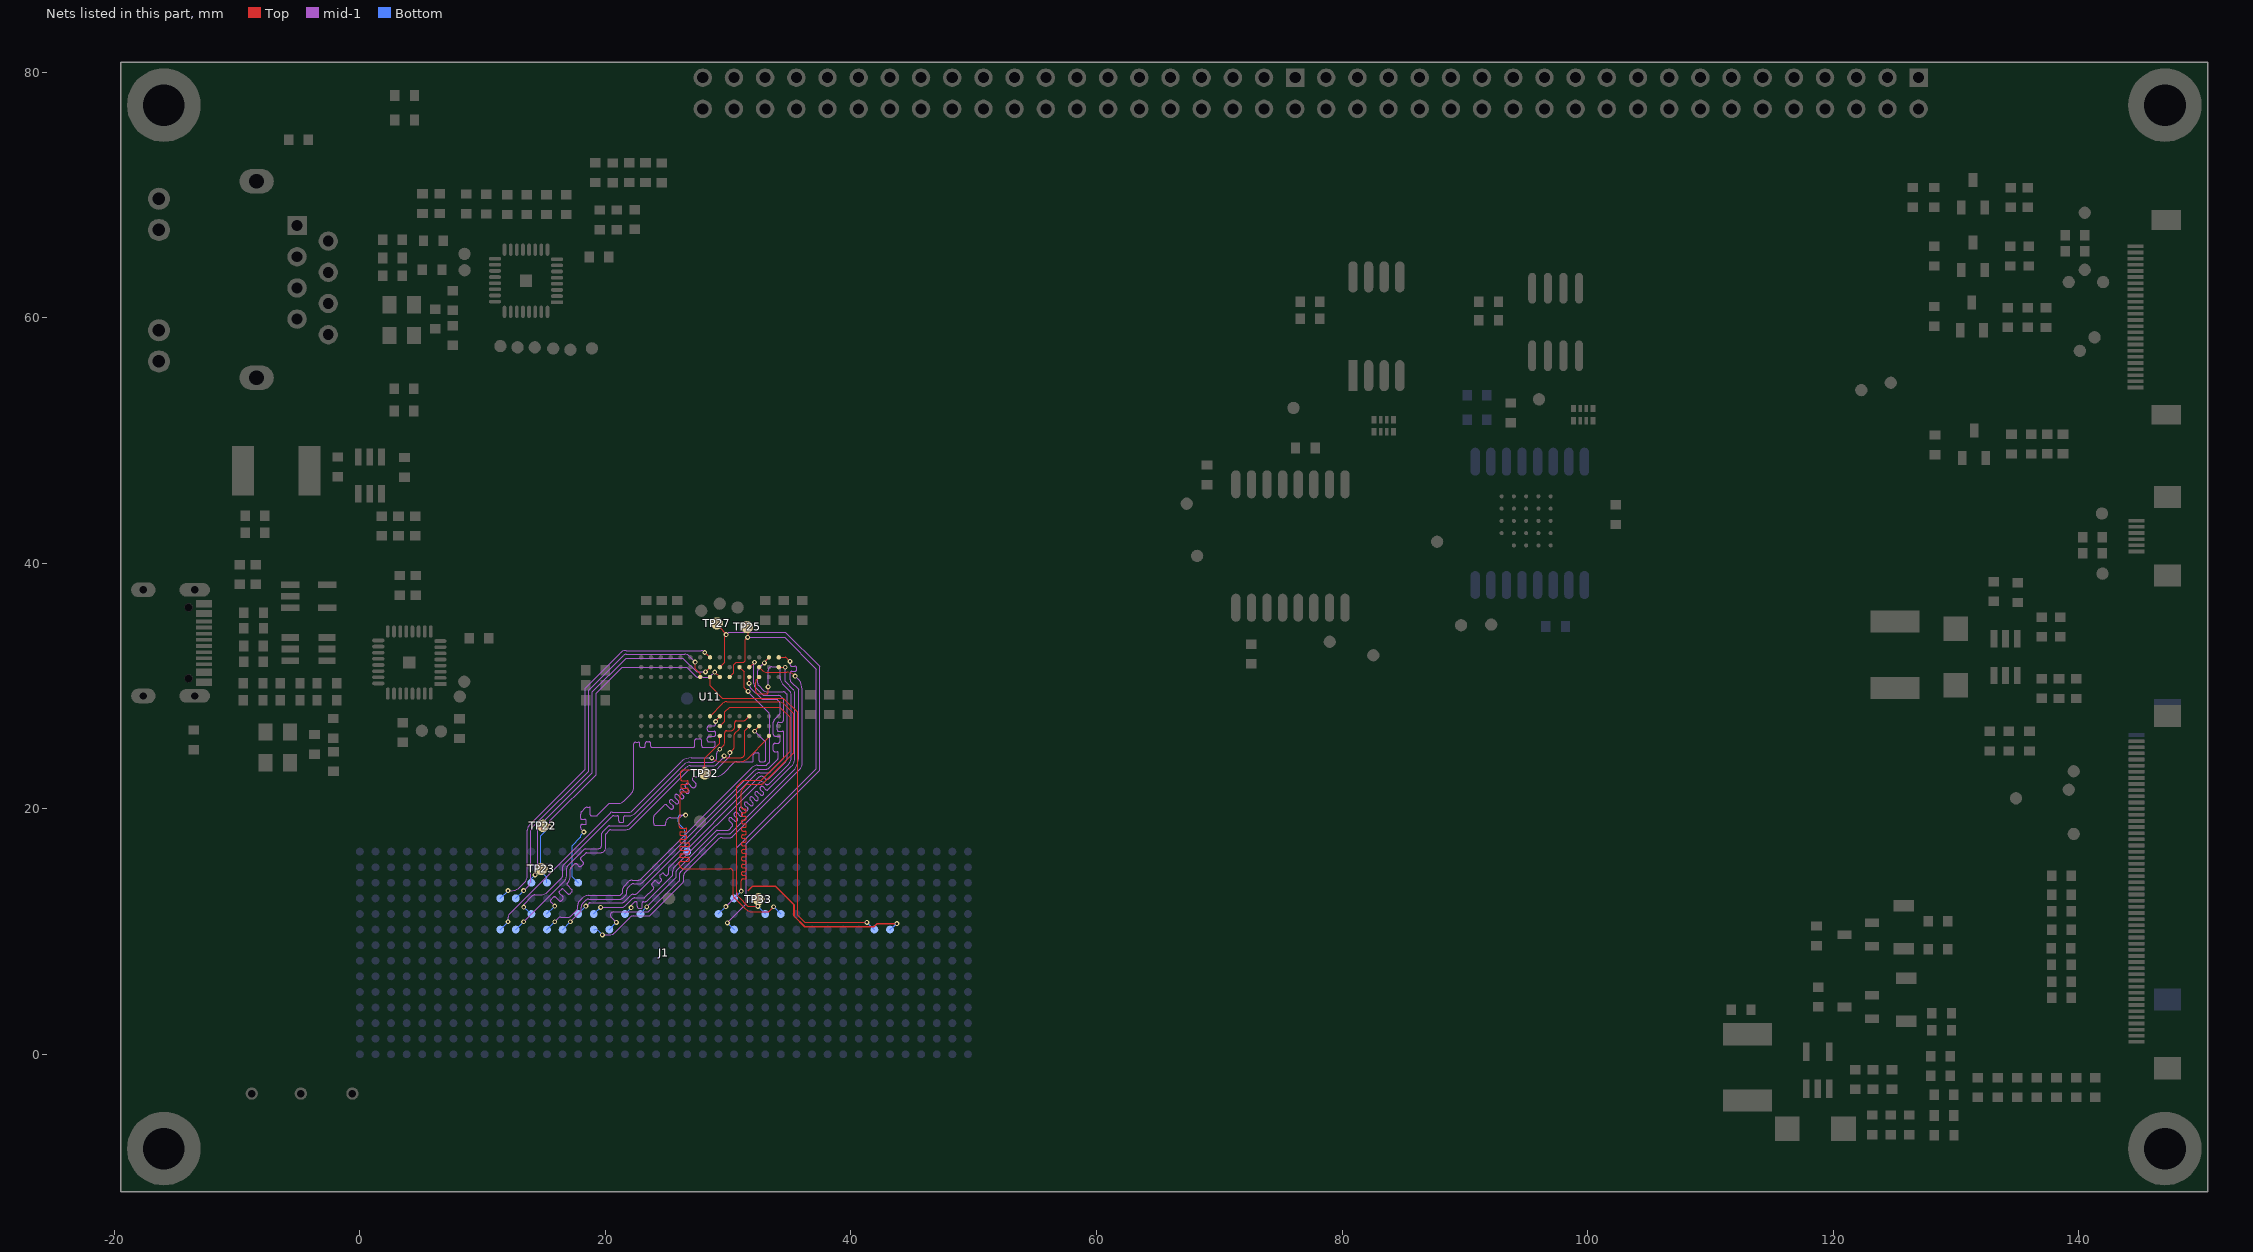
[diagram p0: the nets of this part, all layers, seen from the top]
# Altium PCB MISC105414.PcbDoc (part 9 of 11)
Units mm, origin at the board's own origin, x right, y up, seen from the top; angles counter-clockwise.
Board outline 170 x 92 mm, 6 copper layers (Top, GND, mid-1, mid-2, mid-3, Bottom), stack 1.231 mm thick; 238 components, 304 nets, 1456 pads, 1258 vias.
Unrouted connection lines stored in the file: 57.

## Via types
v1: diameter 0.4, hole 0.2, Top to Bottom, tented top, 618 vias
v2: diameter 0.5, hole 0.3, Top to Bottom, tented top, 522 vias
v3: diameter 0.5, hole 0.3, Top to Bottom, 41 vias
v4: diameter 1, hole 0.5, Top to Bottom, tented top, 36 vias
v5: diameter 0.7, hole 0.4, Top to Bottom, tented top, 34 vias
v6: diameter 1.3, hole 1.3, Top to Bottom, tented top, 3 vias
v7: diameter 4, hole 4, Top to Bottom, tented top, 2 vias
v8: diameter 3.3, hole 3.3, Top to Bottom, tented top, 2 vias

## Nets (pads, with @x,y where several pads share a name; then routed paths per layer and width w, separated by ;. In a path a pad name is that pad's centre, name@x,y a point inside that pad or via, vN(x,y) a via of type N, cw(c..) or ccw(c..) an arc to the next point about the centre after c; other vN are vias at no path point) (continued)
SDR_A9: J1.K26 U11.J3 | length 30.7
  Top w0.1: v1(28.97,27.109) U11.J3@29.32,27.533
  mid-1 w0.1: v1(18.243,18.106) 18.035,18.314 cw(c18.184,18.463) 17.973,18.463 17.973,18.604 cw(c18.094,18.604) 18.094,18.725 18.36,18.725 ccw(c18.36,18.797) 18.432,18.797 18.432,19.034 ccw(c18.334,19.034) 18.334,19.132 18.069,19.132 cw(c18.069,19.228) 17.973,19.228 17.973,19.562 cw(c18.272,19.562) 18.061,19.773 18.363,20.075 cw(c18.525,19.913) 18.525,20.142 18.678,20.142 cw(c18.678,20.044) 18.776,20.044 18.776,19.522 ccw(c18.88,19.522) 18.88,19.417 19.232,19.417 ccw(c19.232,19.57) 19.341,19.462 20.329,20.451 21.108,20.451 ccw(c21.108,21.002) 21.498,20.612 22.075,21.189 ccw(c21.507,21.758) 22.31,21.758 22.31,25.277 cw(c22.469,25.277) 22.469,25.435 22.688,25.435 cw(c22.688,25.326) 22.797,25.326 22.797,25.093 ccw(c22.896,25.093) 22.896,24.994 23.137,24.994 ccw(c23.137,25.094) 23.236,25.094 23.236,25.296 cw(c23.397,25.296) 23.397,25.456 23.546,25.456 cw(c23.546,25.317) 23.686,25.317 23.686,25.109 ccw(c23.8,25.109) 23.8,24.994 27.137,24.994 ccw(c27.137,25.14) 27.283,25.14 27.283,25.567 cw(c27.401,25.567) 27.401,25.685 27.688,25.685 cw(c27.688,25.538) 27.835,25.538 27.835,25.151 ccw(c27.992,25.151) 27.992,24.994 28.751,24.994 ccw(c28.751,25.193) 28.95,25.193 28.95,25.355 ccw(c28.853,25.355) 28.853,25.452 28.419,25.452 cw(c28.419,25.563) 28.308,25.563 28.308,25.762 cw(c28.444,25.762) 28.444,25.898 28.857,25.898 ccw(c28.857,26.011) 28.97,26.011 28.97,26.201 ccw(c28.86,26.201) 28.86,26.312 28.444,26.312 cw(c28.444,26.479) 28.277,26.479 28.277,26.609 cw(c28.425,26.609) 28.425,26.757 28.844,26.757 ccw(c28.844,26.884) 28.97,26.884 v1(28.97,27.109)
  Bottom w0.1: J1.K26@17.78,13.97 17.284,14.466 17.284,17.007 17.957,17.68 ccw(c17.842,17.794) 18.005,17.794 18.005,17.82 cw(c18.12,17.82) 18.038,17.901 v1(18.243,18.106)
SDR_A10: J1.J30 U11.G7 | length 30.9
  Top w0.1: v1(27.307,31.952) 27.307,31.398 27.72,30.985 U11.G7@27.72,30.733
  mid-1 w0.1: v1(13.335,13.335) 13.695,13.695 ccw(c13.13,14.26) 13.929,14.26 13.929,18.236 cw(c14.216,18.236) 14.014,18.439 18.647,23.072 18.647,29.663 21.475,32.491 cw(c21.705,32.261) 21.705,32.587 26.465,32.587 cw(c26.465,32.087) 26.818,32.44 v1(27.307,31.952)
  Bottom w0.1: J1.J30@12.7,12.7 v1(13.335,13.335)
SDR_A11: J1.J31 U11.H9 | length 31.9
  Top w0.1: v1(28.094,32.727) U11.H9@28.52,32.333
  mid-1 w0.1: v1(12.065,13.335) 12.404,13.335 ccw(c12.404,14.175) 12.998,13.581 13.43,14.013 ccw(c12.955,14.488) 13.627,14.488 13.627,18.233 cw(c14.219,18.233) 13.8,18.652 18.346,23.198 18.346,29.816 21.208,32.678 cw(c21.717,32.169) 21.717,32.888 27.792,32.888 cw(c27.792,32.547) 28.033,32.788 v1(28.094,32.727)
  Bottom w0.1: J1.J31@11.43,12.7 v1(12.065,13.335)
SDR_A12: J1.G6 J1.J16 U11.H3 | length 46.1
  Top w0.1: U11.H3@28.52,27.533 29.574,28.586 cw(c29.895,28.265) 29.895,28.72 34.071,28.72 cw(c34.071,28.042) 34.551,28.521 35.268,27.804 cw(c35.064,27.6) 35.353,27.6 35.353,24.658 cw(c35.088,24.658) 35.275,24.471 32.875,22.071 cw(c32.72,22.226) 32.72,22.006 31.644,22.006 ccw(c31.644,21.774) 31.48,21.938 31.182,21.641 ccw(c31.44,21.383) 31.075,21.383 31.075,20.131 ccw(c31.225,20.131) 31.225,19.981 31.338,19.981 cw(c31.338,19.831) 31.488,19.831 cw(c31.338,19.831) 31.338,19.681 31.225,19.681 ccw(c31.225,19.532) 31.075,19.532 ccw(c31.225,19.532) 31.225,19.382 31.338,19.382 cw(c31.338,19.231) 31.488,19.231 cw(c31.338,19.231) 31.338,19.081 31.225,19.081 ccw(c31.225,18.931) 31.075,18.931 ccw(c31.225,18.931) 31.225,18.781 31.338,18.781 cw(c31.338,18.631) 31.488,18.631 cw(c31.338,18.631) 31.338,18.481 31.225,18.481 ccw(c31.225,18.332) 31.075,18.332 ccw(c31.225,18.332) 31.225,18.182 31.338,18.182 cw(c31.338,18.032) 31.488,18.032 cw(c31.338,18.032) 31.338,17.882 31.225,17.881 ccw(c31.225,17.731) 31.075,17.731 ccw(c31.225,17.731) 31.225,17.581 31.338,17.581 cw(c31.338,17.431) 31.488,17.431 cw(c31.338,17.431) 31.338,17.281 31.225,17.281 ccw(c31.225,17.131) 31.075,17.131 ccw(c31.225,17.131) 31.225,16.982 31.338,16.982 cw(c31.338,16.832) 31.488,16.832 cw(c31.338,16.832) 31.338,16.682 31.225,16.681 ccw(c31.225,16.531) 31.075,16.531 ccw(c31.225,16.531) 31.225,16.381 31.338,16.381 cw(c31.338,16.231) 31.488,16.231 cw(c31.338,16.231) 31.338,16.081 31.225,16.081 ccw(c31.225,15.931) 31.075,15.931 ccw(c31.225,15.931) 31.225,15.782 31.338,15.782 cw(c31.338,15.632) 31.488,15.632 cw(c31.338,15.632) 31.338,15.482 31.225,15.482 ccw(c31.225,15.331) 31.075,15.331 ccw(c31.225,15.331) 31.225,15.181 31.338,15.181 cw(c31.338,15.031) 31.488,15.031 cw(c31.338,15.031) 31.338,14.881 31.225,14.881 ccw(c31.225,14.731) 31.075,14.731 ccw(c31.225,14.731) 31.225,14.581 31.338,14.581 cw(c31.338,14.432) 31.488,14.432 cw(c31.338,14.432) 31.338,14.282 31.217,14.282 ccw(c31.217,14.131) 31.067,14.131 v1(31.067,13.287)
  Top w0.127: 31.624,13.316 32.006,13.699 33.843,13.699 35.362,12.18 35.362,11.268 36.247,10.383 41.869,10.383 42.124,10.638 v1(43.746,10.638)
  Bottom w0.1: J1.J16@30.48,12.7 v1(31.067,13.287)
  Bottom w0.127: J1.G6@43.18,10.16 v1(43.746,10.638)
SDR_A13: J1.G7 U11.H7 | length 32
  Top w0.1: U11.H7@28.52,30.733 28.52,30.008 29.508,29.02 34.477,29.02 35.653,27.845 35.653,11.317 36.223,10.747 v1(41.3,10.747)
  Bottom w0.1: v1(41.3,10.747) J1.G7@41.91,10.16
SDR_BA0: J1.K28 TP22.1 U11.J7 | length 29.1
  Top w0.1: v1(28.905,31.129) U11.J7@29.32,30.733
  mid-1 w0.1: v1(15.483,18.53) 15.483,19.026 19.247,22.79 19.247,29.395 21.363,31.511 26.611,31.511 27.297,30.825 ccw(c27.547,31.075) 27.547,30.721 28.305,30.721 ccw(c28.305,31.184) 28.633,30.857 v1(28.905,31.129)
  Bottom w0.1: J1.K28@15.24,13.97 15.24,14.418 14.741,14.917 14.741,17.787 v1(15.483,18.53)
SDR_BA1: J1.K29 TP23.1 U11.H8 | length 29
  Top w0.1: v1(28.153,31.148) U11.H8@28.52,31.533
  mid-1 w0.1: v1(14.28,14.614) 14.363,14.698 14.493,14.828 14.493,18.485 18.947,22.939 18.947,29.537 21.689,32.28 26.315,32.28 27.447,31.148 v1(28.153,31.148)
  Bottom w0.1: J1.K29@13.97,13.97 13.97,14.305 v1(14.28,14.614)
SDR_CAS: J1.H17 TP25.1 U11.K7 | length 34.9
  Top w0.1: U11.K7@30.12,30.733 30.468,31.081 30.468,31.736 30.665,31.933 31.263,31.933 31.377,32.046 31.377,33.753 v1(31.576,33.952) TP25.1@31.545,34.807
  mid-1 w0.1: v1(29.807,12.022) 30.714,12.928 30.714,16.815 37.171,23.273 37.171,31.369 34.588,33.952 v1(31.576,33.952)
  Bottom w0.1: J1.H17@29.21,11.43 v1(29.807,12.022)
SDR_CKE: J1.H14 TP33.1 U11.J2 | length 27.2
  Top w0.1: U11.J2@29.32,26.733 29.314,26.734 29.72,27.14 29.72,27.896 30.112,28.288 34.2,28.288 35.05,27.437 35.05,24.67 32.78,22.4 cw(c32.554,22.626) 32.554,22.306 31.215,22.306 30.717,21.809 30.717,13.182 ccw(c31.28,13.182) 30.882,12.783 31.568,12.097 ccw(c31.697,12.227) 31.697,12.044 v1(32.421,12.044)
  Bottom w0.1: v1(32.421,12.044) 32.416,12.039 J1.H14@33.02,11.43
SDR_CLK: J1.H13 TP32.1 U11.J1 | length 32.3
  Top w0.1: U11.J1@29.32,25.933 29.32,25.347 28.093,24.121 28.093,23.483 27.789,23.179 26.283,23.179 26.127,23.023 26.127,22.43 ccw(c26.277,22.43) 26.277,22.28 26.65,22.28 cw(c26.65,22.171) 26.758,22.171 26.758,22.114 cw(c26.624,22.114) 26.624,21.98 26.277,21.98 ccw(c26.277,21.83) 26.127,21.83 ccw(c26.277,21.83) 26.277,21.68 26.644,21.68 cw(c26.644,21.557) 26.767,21.557 26.767,21.493 cw(c26.653,21.493) 26.653,21.38 26.277,21.38 ccw(c26.277,21.23) 26.127,21.23 26.114,21.216 26.114,19.373 26.004,19.264 26.004,18.582 ccw(c26.154,18.582) 26.154,18.432 26.534,18.432 cw(c26.534,18.328) 26.639,18.328 26.639,18.246 cw(c26.525,18.246) 26.525,18.132 26.194,18.132 ccw(c26.194,17.982) 26.044,17.982 ccw(c26.194,17.982) 26.194,17.832 26.527,17.832 cw(c26.527,17.739) 26.62,17.739 26.62,17.643 cw(c26.51,17.643) 26.51,17.532 26.194,17.532 ccw(c26.194,17.382) 26.044,17.382 ccw(c26.194,17.382) 26.194,17.232 26.704,17.232 cw(c26.704,17.082) 26.854,17.082 cw(c26.704,17.082) 26.704,16.932 26.194,16.932 ccw(c26.194,16.782) 26.044,16.782 ccw(c26.194,16.782) 26.194,16.632 26.704,16.632 cw(c26.704,16.482) 26.854,16.482 cw(c26.704,16.482) 26.704,16.332 26.194,16.332 ccw(c26.194,16.182) 26.044,16.182 ccw(c26.194,16.182) 26.194,16.032 26.704,16.032 cw(c26.704,15.882) 26.854,15.882 cw(c26.704,15.882) 26.704,15.732 26.182,15.732 ccw(c26.182,15.582) 26.032,15.582 26.032,15.435 ccw(c26.337,15.435) 26.337,15.13 30.11,15.13 cw(c30.11,14.823) 30.416,14.823 30.416,12.953 ccw(c30.728,12.953) 30.507,12.732 31.404,11.835 ccw(c31.933,12.364) 31.933,11.616 33.207,11.616 ccw(c33.207,11.841) 33.366,11.682 v1(33.7,12.017)
  Bottom w0.1: v1(33.7,12.017) J1.H13@34.29,11.43
SDR_CS: J1.G16 TP27.1 U11.J8 | length 37.7
  Top w0.1: TP27.1@29.077,35.099 v1(29.828,34.179) 29.713,34.064 29.713,31.926 U11.J8@29.32,31.533
  mid-1 w0.1: v1(29.828,34.179) 30.046,34.397 34.663,34.397 37.471,31.589 37.471,23.148 31.469,17.146 31.469,12.248 v1(29.932,10.711)
  Bottom w0.1: v1(29.932,10.711) J1.G16@30.48,10.16
SDR_D0: J1.H22 U11.R8 | length 33.3
  Top w0.1: U11.R8@34.12,31.533 34.128,31.525 v1(34.649,31.525)
  mid-1 w0.1: v1(23.365,12.004) 25.7,14.339 ccw(c25.54,14.5) 25.767,14.5 25.767,14.892 cw(c25.901,14.892) 25.806,14.987 29.049,18.23 cw(c29.113,18.166) 29.113,18.257 29.961,18.257 ccw(c29.961,18.41) 30.069,18.301 30.33,18.563 ccw(c30.224,18.669) 30.374,18.669 ccw(c30.224,18.669) 30.33,18.775 30.086,19.019 cw(c30.192,19.125) 30.042,19.125 cw(c30.192,19.125) 30.086,19.231 cw(c30.192,19.125) 30.298,19.231 30.516,19.014 ccw(c30.622,19.12) 30.772,19.12 ccw(c30.622,19.12) 30.728,19.226 30.511,19.443 cw(c30.617,19.55) 30.467,19.55 cw(c30.617,19.55) 30.723,19.656 30.94,19.438 ccw(c31.046,19.544) 31.196,19.544 ccw(c31.046,19.544) 31.152,19.65 30.935,19.868 cw(c31.041,19.974) 30.891,19.974 cw(c31.041,19.974) 31.147,20.08 31.364,19.862 ccw(c31.47,19.969) 31.62,19.969 ccw(c31.47,19.969) 31.576,20.075 31.359,20.292 cw(c31.465,20.398) 31.315,20.398 cw(c31.465,20.398) 31.571,20.504 31.789,20.287 ccw(c31.895,20.393) 32.045,20.393 ccw(c31.895,20.393) 32.001,20.499 31.783,20.716 cw(c31.889,20.822) 31.739,20.822 cw(c31.889,20.822) 31.995,20.928 32.213,20.711 ccw(c32.319,20.817) 32.469,20.817 ccw(c32.319,20.817) 32.425,20.923 32.208,21.141 cw(c32.314,21.247) 32.164,21.247 cw(c32.314,21.247) 32.42,21.353 32.637,21.135 ccw(c32.743,21.241) 32.893,21.241 ccw(c32.743,21.241) 32.849,21.347 32.632,21.565 cw(c32.738,21.671) 32.588,21.671 cw(c32.738,21.671) 32.844,21.777 33.061,21.56 ccw(c33.167,21.666) 33.23,21.529 35.143,23.442 ccw(c34.456,24.129) 35.428,24.129 35.428,29.381 ccw(c34.913,29.381) 35.277,29.745 34.649,30.373 v1(34.649,31.525)
  Bottom w0.1: J1.H22@22.86,11.43 22.86,11.499 v1(23.365,12.004)
SDR_D1: J1.H23 U11.N7 | length 33.4
  Top w0.1: U11.N7@32.52,30.733 32.315,30.528 ccw(c32.518,30.325) 32.231,30.325 32.231,29.607 ccw(c32.474,29.607) 32.474,29.364 33.135,29.364 ccw(c33.135,29.48) 33.251,29.48 v1(33.251,29.93)
  mid-1 w0.1: v1(22.1,11.95) 22.1,12.094 cw(c22.23,12.094) 22.138,12.185 22.329,12.376 cw(c22.488,12.216) 22.488,12.442 22.496,12.442 cw(c22.496,12.349) 22.588,12.349 22.588,12.044 ccw(c22.74,12.044) 22.74,11.892 22.899,11.892 ccw(c22.899,12.007) 23.014,12.007 23.014,12.349 cw(c23.108,12.349) 23.108,12.442 23.253,12.442 ccw(c23.253,12.589) 23.356,12.485 25.465,14.594 25.465,14.921 cw(c25.846,14.921) 25.576,15.19 ; 25.577,15.19 32.472,22.086 cw(c32.716,21.842) 32.96,22.086 33.03,22.015 ccw(c33.161,22.146) 33.292,22.015 34.914,23.637 ccw(c34.397,24.154) 35.128,24.154 35.128,29.333 ccw(c34.799,29.333) 35.031,29.566 34.412,30.186 cw(c34.809,30.583) 34.247,30.583 34.247,31.355 ccw(c34.034,31.355) 34.034,31.568 33.547,31.568 ccw(c33.547,31.273) 33.251,31.273 v1(33.251,29.93)
  Bottom w0.1: J1.H23@21.59,11.43 v1(22.1,11.95)
SDR_D2: J1.G24 U11.R9 | length 33
  Top w0.1: U11.R9@34.12,32.333 34.635,32.333 cw(c34.635,32.141) 34.77,32.277 v1(35.035,32.012)
  mid-1 w0.1: v1(20.9,10.75) 20.47,11.18 cw(c20.64,11.35) 20.399,11.35 cw(c20.64,11.35) 20.64,11.591 23.491,11.591 26.02,14.12 ccw(c25.896,14.243) 26.071,14.243 26.071,14.747 cw(c26.263,14.747) 26.127,14.883 29.162,17.918 cw(c29.256,17.823) 29.256,17.957 30.082,17.957 ccw(c30.082,18.118) 30.196,18.004 35.338,23.146 ccw(c34.397,24.087) 35.728,24.087 35.728,29.719 35.116,30.331 cw(c35.312,30.526) 35.035,30.526 35.035,31.043 cw(c35.188,31.043) 35.188,31.196 35.436,31.196 ccw(c35.436,31.342) 35.582,31.342 35.582,31.456 ccw(c35.413,31.456) 35.413,31.624 35.142,31.624 cw(c35.142,31.731) 35.035,31.731 v1(35.035,32.012)
  Bottom w0.1: J1.G24@20.32,10.16 v1(20.9,10.75)
SDR_D3: J1.G25 U11.N8 | length 33.8
  Top w0.1: U11.N8@32.52,31.533 32.764,31.289 ccw(c33.15,31.675) 33.15,31.129 34.771,31.129 cw(c34.771,30.25) 35.393,30.872 v1(35.457,30.808)
  mid-1 w0.1: v1(19.747,9.732) 20.366,9.732 ccw(c20.366,10.295) 20.763,9.897 22.035,11.168 cw(c22.269,10.934) 22.269,11.265 23.463,11.265 ccw(c23.463,11.575) 23.682,11.356 26.297,13.971 ccw(c26.112,14.156) 26.373,14.156 26.373,14.575 cw(c26.685,14.575) 26.465,14.796 29.185,17.516 cw(c29.517,17.183) 29.517,17.654 30.183,17.654 ccw(c30.183,17.873) 30.338,17.718 35.832,23.212 ccw(c35.358,23.685) 36.028,23.685 36.028,29.728 ccw(c34.8,29.728) 35.668,30.597 v1(35.457,30.808)
  Bottom w0.1: J1.G25@19.05,10.16 19.126,10.16 cw(c19.126,9.694) 19.456,10.024 v1(19.747,9.732)
SDR_D4: J1.H25 U11.P9 | length 33.2
  Top w0.1: v1(32.949,31.885) U11.P9@33.32,32.333
  mid-1 w0.1: v1(19.615,11.964) 21.301,11.964 ccw(c21.301,12.427) 21.628,12.1 22.187,12.659 cw(c22.388,12.458) 22.388,12.742 23.14,12.742 ccw(c23.14,12.86) 23.224,12.777 23.927,13.48 ccw(c23.858,13.549) 23.956,13.549 ccw(c23.858,13.549) 23.927,13.618 23.782,13.763 cw(c23.852,13.833) 23.753,13.833 cw(c23.852,13.833) 23.782,13.903 ; 23.782,13.903 23.985,14.106 cw(c24.058,14.034) 24.13,14.106 24.269,13.967 ; 24.27,13.966 ccw(c24.342,14.039) 24.413,13.966 ; 24.414,13.967 24.565,14.118 ccw(c24.49,14.194) 24.597,14.194 ccw(c24.49,14.194) 24.565,14.27 24.446,14.389 cw(c24.535,14.478) 24.409,14.478 cw(c24.535,14.478) 24.446,14.567 24.599,14.72 cw(c24.679,14.641) 24.758,14.72 24.885,14.593 ccw(c24.963,14.67) 25.04,14.593 25.125,14.678 ccw(c25.039,14.764) 25.161,14.764 25.161,15.212 32.496,22.548 cw(c32.71,22.334) 32.923,22.548 33.025,22.446 ccw(c33.162,22.582) 33.298,22.446 34.697,23.844 ccw(c34.38,24.161) 34.828,24.161 34.828,29.233 ccw(c34.69,29.233) 34.787,29.33 34.664,29.454 ; v1(32.949,31.885) 32.456,31.392 ccw(c32.602,31.246) 32.396,31.246 32.396,30.237 ccw(c32.67,30.237) 32.476,30.043 32.854,29.664 ccw(c33.18,29.99) 33.18,29.53 34.481,29.53 cw(c34.481,29.271) 34.664,29.454
  Bottom w0.1: J1.H25@19.05,11.43 19.6,11.98 v1(19.615,11.964)
SDR_D5: J1.H26 U11.M8 | length 32.9
  Top w0.1: U11.M8@31.72,31.533 v1(32.144,31.932)
  mid-1 w0.1: v1(18.415,12.065) 18.63,12.28 cw(c18.757,12.153) 18.757,12.333 21.311,12.333 ccw(c21.311,12.637) 21.526,12.422 22.061,12.957 cw(c22.283,12.735) 22.283,13.049 22.453,13.049 ccw(c22.453,13.172) 22.54,13.085 32.255,22.8 cw(c32.584,22.471) 32.584,22.937 33.26,22.937 ccw(c33.26,23.189) 33.438,23.01 34.464,24.036 ccw(c34.31,24.19) 34.528,24.19 34.528,26.2 ccw(c34.412,26.2) 34.412,26.316 34.117,26.316 cw(c34.117,26.449) 33.983,26.449 33.983,26.902 cw(c34.12,26.902) 34.12,27.039 34.31,27.039 ccw(c34.31,27.256) 34.528,27.256 34.528,28.83 ccw(c34.333,28.83) 34.471,28.967 34.309,29.129 ccw(c34.068,28.887) 34.068,29.229 32.977,29.229 cw(c32.977,29.499) 32.787,29.308 32.238,29.857 ; v1(32.144,31.932) 32.082,31.87 32.082,30.232 ccw(c32.613,30.232) 32.238,29.857
  Bottom w0.1: J1.H26@17.78,11.43 v1(18.415,12.065)
SDR_D6: J1.G27 U11.M7 | length 33.5
  Top w0.1: v1(31.702,30.217) 31.72,30.234 U11.M7@31.72,30.733
  mid-1 w0.1: v1(17.145,10.795) 17.942,11.592 ccw(c17.731,11.803) 18.029,11.803 18.029,11.99 cw(c18.474,11.99) 18.159,12.304 18.385,12.53 cw(c18.637,12.279) 18.637,12.635 21.181,12.635 ccw(c21.181,12.957) 21.409,12.729 21.694,13.014 ccw(c21.616,13.092) 21.726,13.092 21.726,13.347 cw(c22.027,13.347) 21.814,13.56 22.04,13.786 cw(c22.302,13.523) 22.302,13.894 22.796,13.894 ccw(c22.796,14.202) 23.013,13.984 32.136,23.107 cw(c32.45,22.792) 32.45,23.237 33.15,23.237 ccw(c33.15,23.455) 33.304,23.301 34.035,24.031 ccw(c33.883,24.183) 34.098,24.183 34.098,24.535 ccw(c33.979,24.535) 33.979,24.654 33.775,24.654 cw(c33.775,24.746) 33.683,24.746 33.683,25.2 cw(c33.825,25.2) 33.825,25.342 34.063,25.342 ccw(c34.063,25.507) 34.228,25.507 34.228,25.806 ccw(c34.114,25.806) 34.114,25.92 33.834,25.92 cw(c33.834,26.072) 33.683,26.072 33.683,27.053 cw(c33.957,27.053) 33.763,27.247 34.134,27.618 ccw(c33.909,27.844) 34.228,27.844 34.228,28.593 ccw(c34.03,28.593) 34.17,28.733 34.052,28.851 ccw(c33.908,28.708) 33.908,28.911 32.877,28.911 cw(c32.877,29.194) 32.676,28.994 31.804,29.867 cw(c31.977,30.04) 31.732,30.04 31.732,30.217 v1(31.702,30.217)
  Bottom w0.1: J1.G27@16.51,10.16 v1(17.145,10.795)
SDR_D7: J1.G28 U11.L8 | length 32.9
  Top w0.1: U11.L8@30.92,31.533 31.3,31.153 31.3,29.875 v1(31.619,29.556)
  mid-1 w0.1: v1(15.875,10.795) 16.172,11.092 cw(c16.377,10.887) 16.377,11.177 17.014,11.177 ccw(c17.014,11.39) 17.164,11.239 17.677,11.752 ccw(c17.552,11.877) 17.729,11.877 17.729,12.131 cw(c18.133,12.131) 17.847,12.416 18.204,12.774 cw(c18.593,12.385) 18.593,12.935 21.12,12.935 ccw(c21.12,13.105) 21.24,12.985 ; 21.24,12.985 21.386,13.131 ccw(c21.293,13.225) 21.425,13.225 21.425,13.467 cw(c21.737,13.467) 21.517,13.688 21.911,14.082 cw(c22.184,13.809) 22.184,14.195 22.716,14.195 ccw(c22.716,14.396) 22.859,14.254 31.977,23.372 cw(c32.374,22.975) 32.374,23.537 33.015,23.537 ccw(c33.015,23.778) 33.186,23.607 33.318,23.74 ccw(c33.173,23.885) 33.378,23.885 33.378,27.616 ccw(c33.039,27.616) 33.279,27.856 31.595,29.54 31.612,29.558 31.615,29.56 v1(31.619,29.556)
  Bottom w0.1: J1.G28@15.24,10.16 v1(15.875,10.795)
SDR_D8: J1.H28 U11.L2 | length 28.1
  Top w0.1: v1(30.139,24.576) 30.414,24.85 ccw(c30.196,25.068) 30.504,25.068 30.504,26.037 cw(c30.643,26.037) 30.545,26.135 30.896,26.487 ccw(c30.839,26.544) 30.92,26.544 U11.L2@30.92,26.733
  mid-1 w0.1: 15.728,12.764 15.571,12.606 ccw(c15.689,12.488) 15.521,12.488 ccw(c15.689,12.488) 15.571,12.369 v1(15.875,12.065) ; 15.729,12.764 15.754,12.788 cw(c15.851,12.691) 15.948,12.788 16.201,12.536 ccw(c16.326,12.661) 16.451,12.536 16.522,12.607 ccw(c16.399,12.73) 16.573,12.73 ccw(c16.399,12.73) 16.522,12.853 16.246,13.129 cw(c16.322,13.205) 16.215,13.205 cw(c16.322,13.205) 16.246,13.281 16.425,13.46 cw(c16.487,13.397) 16.549,13.46 16.922,13.086 ccw(c17.021,13.185) 17.119,13.086 17.268,13.235 ccw(c17.178,13.325) 17.305,13.325 ccw(c17.178,13.325) 17.268,13.415 16.891,13.792 cw(c16.957,13.859) 16.863,13.859 cw(c16.957,13.859) 16.891,13.926 16.894,13.929 ccw(c16.31,14.512) 17.135,14.512 17.135,15.071 cw(c17.287,15.071) 17.18,15.178 17.475,15.474 cw(c17.581,15.368) 17.687,15.474 17.825,15.336 ccw(c17.929,15.44) 18.032,15.336 18.195,15.498 ccw(c18.123,15.57) 18.225,15.57 ccw(c18.123,15.57) 18.195,15.642 18.004,15.834 cw(c18.088,15.918) 17.969,15.918 cw(c18.088,15.918) 18.004,16.002 18.386,16.384 ; 18.386,16.384 cw(c18.481,16.289) 18.481,16.423 19.575,16.423 ccw(c19.575,16.882) 20.033,16.882 20.033,17.904 cw(c20.146,17.904) 20.066,17.983 20.356,18.273 cw(c20.435,18.194) 20.435,18.305 21.7,18.305 ccw(c21.7,18.883) 22.108,18.475 26.757,23.124 cw(c26.926,22.954) 26.926,23.194 28.818,23.194 ccw(c28.818,23.806) 29.251,23.373 30.063,24.185 ccw(c29.879,24.369) 30.139,24.369 v1(30.139,24.576)
  Bottom w0.1: J1.H28@15.24,11.43 v1(15.875,12.065)
SDR_D9: J1.H29 U11.M3 | length 28.2
  Top w0.1: v1(29.313,24.844) 29.606,25.137 ccw(c29.366,25.376) 29.705,25.376 29.705,26.187 cw(c29.867,26.187) 29.867,26.349 30.194,26.349 ccw(c30.194,26.671) 30.422,26.443 30.462,26.483 ccw(c30.283,26.661) 30.536,26.661 30.536,27.023 cw(c30.674,27.023) 30.674,27.162 31.22,27.162 ccw(c31.22,27.472) 31.44,27.253 U11.M3@31.72,27.533
  mid-1 w0.1: v1(13.347,11.988) 13.347,12.128 cw(c13.508,12.128) 13.394,12.241 14.059,12.906 cw(c14.238,12.727) 14.238,12.98 14.717,12.98 ccw(c14.717,13.76) 15.268,13.208 16.444,14.384 ; 16.445,14.384 ccw(c16.24,14.589) 16.529,14.589 16.529,15.292 cw(c16.732,15.292) 16.588,15.435 20.508,19.355 cw(c20.677,19.186) 20.677,19.425 20.98,19.425 cw(c20.98,19.328) 21.076,19.328 21.076,19.012 ccw(c21.181,19.012) 21.181,18.907 21.423,18.907 ccw(c21.423,18.992) 21.508,18.992 21.508,19.34 cw(c21.593,19.34) 21.593,19.425 21.945,19.425 ccw(c21.945,20.062) 22.396,19.611 26.388,23.603 cw(c26.858,23.133) 26.858,23.798 28.713,23.798 ccw(c28.713,24.071) 28.906,23.878 28.997,23.968 ccw(c28.86,24.105) 29.053,24.105 29.053,24.519 cw(c29.209,24.519) 29.099,24.63 v1(29.313,24.844)
  Bottom w0.1: v1(13.347,11.988) 13.348,11.975 13.957,11.429 J1.H29@13.97,11.43
SDR_D10: J1.G30 U11.M2 | length 28.3
  Top w0.1: v1(29.67,24.306) 29.768,24.208 ccw(c29.886,24.327) 29.886,24.159 31.016,24.159 ccw(c31.016,24.502) 31.358,24.502 31.358,26.371 U11.M2@31.72,26.733
  mid-1 w0.1: v1(13.335,10.795) 16.678,14.138 ccw(c16.298,14.518) 16.835,14.518 16.835,15.173 cw(c17.04,15.173) 16.895,15.318 18.246,16.669 cw(c18.378,16.537) 18.378,16.723 19.346,16.723 ccw(c19.346,17.096) 19.719,17.096 19.719,17.992 cw(c19.883,17.992) 19.767,18.108 20.215,18.556 cw(c20.335,18.435) 20.335,18.605 21.669,18.605 ccw(c21.669,18.957) 21.917,18.709 26.547,23.338 cw(c26.923,22.962) 26.923,23.494 28.703,23.494 ccw(c28.703,24.084) 29.12,23.667 29.67,24.217 v1(29.67,24.306)
  Bottom w0.1: J1.G30@12.7,10.16 v1(13.335,10.795)
SDR_D11: J1.G31 U11.P1 | length 28.9
  Top w0.1: v1@28.665,24.147 ccw(c29.387,24.869) 29.387,23.848 30.994,23.848 ccw(c30.994,24.673) 31.577,24.09 33.254,25.767 ccw(c33.096,25.925) 33.32,25.925 U11.P1@33.32,25.933
  mid-1 w0.1: v1(12.065,10.795) 12.065,11.16 cw(c12.49,11.16) 12.19,11.461 20.379,19.651 cw(c20.561,19.469) 20.561,19.726 21.926,19.726 ccw(c21.926,20.113) 22.2,19.839 26.178,23.818 cw(c26.975,23.021) 26.975,24.148 v1(28.664,24.148)
  Bottom w0.1: J1.G31@11.43,10.16 v1(12.065,10.795)
SDR_D12: J1.M19 U11.N2 | length 28.5
  Top w0.1: v1(32.151,26.316) 32.151,26.364 U11.N2@32.52,26.733
  mid-1 w0.1: v1(26.533,19.489) 26.353,19.489 ccw(c26.353,19.294) 26.214,19.432 26.11,19.328 cw(c26.002,19.436) 26.002,19.283 25.326,19.283 ccw(c25.326,18.865) 24.909,18.865 24.909,18.761 cw(c24.797,18.761) 24.797,18.649 24.085,18.649 cw(c24.085,18.808) 23.926,18.808 23.926,19.354 cw(c24.112,19.354) 23.98,19.486 24.797,20.302 cw(c24.903,20.196) 25.009,20.302 25.296,20.014 ccw(c25.403,20.12) 25.553,20.12 ccw(c25.403,20.12) 25.509,20.226 25.247,20.488 cw(c25.353,20.594) 25.203,20.594 cw(c25.353,20.594) 25.459,20.7 25.721,20.438 ccw(c25.827,20.545) 25.977,20.545 ccw(c25.827,20.545) 25.933,20.651 25.672,20.912 cw(c25.778,21.018) 25.628,21.018 cw(c25.778,21.018) 25.884,21.124 26.145,20.863 ccw(c26.251,20.969) 26.401,20.969 ccw(c26.251,20.969) 26.357,21.075 26.096,21.336 cw(c26.202,21.442) 26.052,21.442 cw(c26.202,21.442) 26.308,21.548 26.569,21.287 ccw(c26.675,21.393) 26.825,21.393 ccw(c26.675,21.393) 26.781,21.499 26.52,21.76 cw(c26.626,21.867) 26.476,21.867 cw(c26.626,21.867) 26.52,21.973 26.589,22.042 cw(c26.679,21.952) 26.769,22.042 27.039,21.771 ccw(c27.169,21.901) 27.298,21.771 27.331,21.804 ccw(c27.182,21.954) 27.393,21.954 ccw(c27.182,21.954) 27.331,22.104 27.109,22.326 cw(c27.22,22.437) 27.063,22.437 cw(c27.22,22.437) 27.22,22.594 28.838,22.594 ccw(c28.838,23.759) 29.662,22.935 30.466,23.739 cw(c30.706,23.499) 30.706,23.839 31.973,23.839 ccw(c31.973,23.924) 32.058,23.924 32.058,24.391 cw(c32.221,24.391) 32.221,24.554 32.402,24.554 cw(c32.402,24.426) 32.531,24.426 32.531,23.917 ccw(c32.61,23.917) 32.61,23.839 32.902,23.839 ccw(c32.902,24.015) 33.078,24.015 33.078,25.259 ccw(c32.764,25.259) 32.986,25.481 v1(32.151,26.316)
  Bottom w0.1: v1(26.533,19.489) 26.127,19.489 ccw(c26.127,19.304) 25.942,19.304 25.942,18.926 ccw(c26.221,18.926) 26.024,18.728 26.368,18.384 cw(c26.039,18.055) 26.504,18.055 26.504,16.676 J1.M19@26.67,16.51